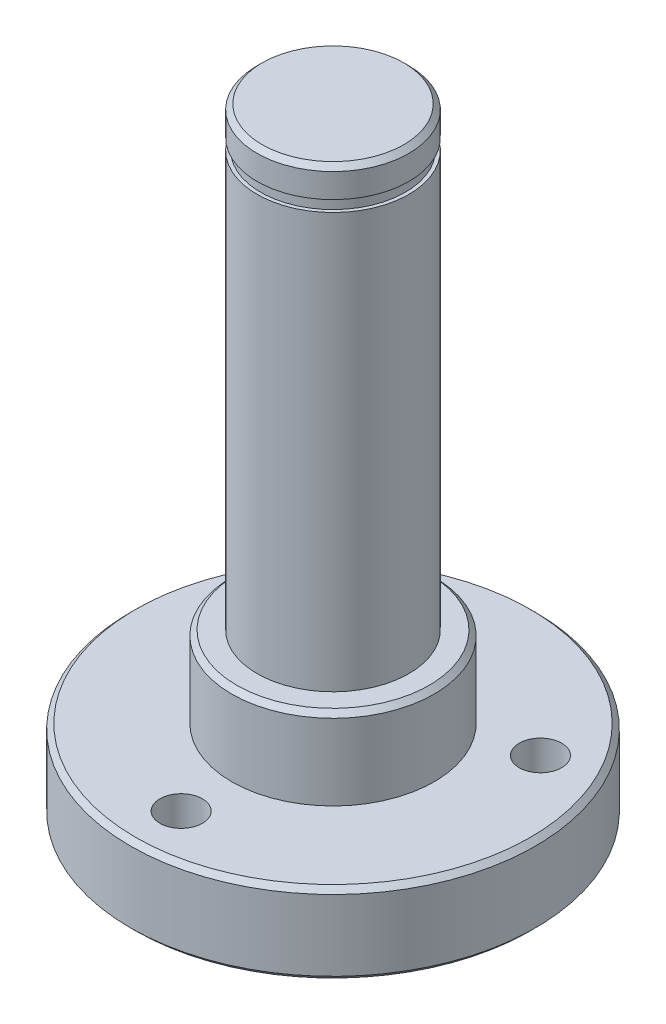
SolidWorks part; units mm, degrees
ref_plane "前视基准面" through (0, 0, 0) normal (0, 0, 1) x (1, 0, 0)
ref_plane "上视基准面" through (0, 0, 0) normal (0, 1, 0) x (1, 0, 0)
ref_plane "右视基准面" through (0, 0, 0) normal (1, 0, 0) x (0, 0, -1)
sketch "草图1" plane through (0, 0, 0) normal (0, 1, 0) x (1, 0, 0)
  circle A0 centre (0, 0) radius 20
  dimension "D1" = 40
extrude "凸台-拉伸1" add sketch "草图1" along normal mid plane 8
sketch "草图2" plane through (0, 4, 0) normal (0, 1, 0) x (1, 0, 0)
  circle A0 centre (0, 0) radius 10
  dimension "D1" = 20
extrude "凸台-拉伸2" add sketch "草图2" along normal blind 8
sketch "草图3" plane through (0, 12, 0) normal (0, 1, 0) x (1, 0, 0)
  circle A0 centre (0, 0) radius 7.5
  dimension "D1" = 15
extrude "凸台-拉伸3" add sketch "草图3" along normal blind 45
sketch "草图4" plane through (0, 0, 0) normal (1, 0, 0) x (0, 0, -1)
  line L0 (7.5, 12) -> (7.5, 57) construction
  line L1 (7.5, 54.1) -> (7.15, 54.1)
  line L2 (7.5, 54.1) -> (7.5, 53)
  line L3 (7.5, 53) -> (7.15, 53)
  line L4 (7.15, 54.1) -> (7.15, 53)
  line L5 (10, 12) -> (-10, 12) construction
  line L6 (0, 0) -> (0, 66.771) construction
  dimension "D1" = 41
  dimension "D2" = 1.1
  dimension "D3" = 0.35
revolve "切除-旋转1" cut sketch "草图4" angle 360 about L6
hole_wizard "M5 螺纹孔1" positions "草图6" profile "草图5" tap size "M5" standard "ISO" end condition through all
sketch "草图6" plane through (0, 4, 0) normal (0, 1, 0) x (1, 0, 0)
  line L0 (0, 0) -> (0, -23.4034) construction
  line L2 (0, 0) -> (37.132, 21.4382) construction
  line L4 (0, 0) -> (-20.8587, 12.0428) construction
  circle A0 centre (0, 0) radius 15 construction
  point P4 (-12.9904, 7.5)
  point P13 (12.9904, 7.5)
  point P14 (0, -15)
  dimension "D1" = 30
  dimension "D3" = 120
  dimension "D4" = 120
  dimension "D2" = 3
sketch "草图5" plane through (-12.9904, 4, -7.5) normal (1, 0, 0) x (0, 0, 1)
  line L0 (0, 0) -> (0, 8)
  line L1 (0, 8) -> (2.1, 8)
  line L2 (2.1, 8) -> (2.1, 0)
  line L5 (2.1, 0) -> (0, 0)
  line L11 (0, -6.35) -> (0, 107.95) construction
  dimension "通孔螺纹孔钻头直径" = 4.2
  dimension "通孔螺纹孔钻头深度" = 8
cosmetic thread "孔螺蚊线1" parameters "D2"=5
cosmetic thread "孔螺蚊线2" parameters "D2"=5
cosmetic thread "孔螺蚊线3" parameters "D2"=5
chamfer "倒角1" distance 0.5 angle 45 2 edges at (0, 57, 7.5) (0, 12, 10)
chamfer "倒角2" distance 0.5 angle 45 2 edges at (0, -4, 20) (0, 4, 20)
